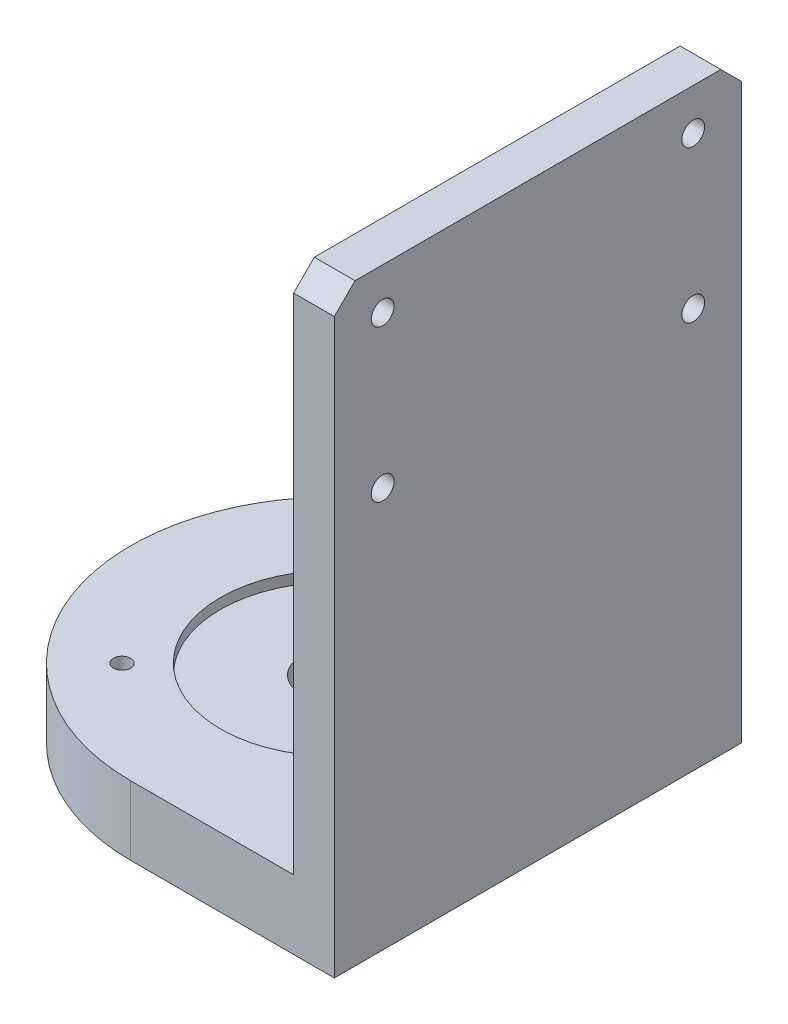
SolidWorks part; units mm, degrees
ref_plane "Front Plane" through (0, 0, 0) normal (0, 0, 1) x (1, 0, 0)
ref_plane "Top Plane" through (0, 0, 0) normal (0, 1, 0) x (1, 0, 0)
ref_plane "Right Plane" through (0, 0, 0) normal (1, 0, 0) x (0, 0, -1)
sketch "Sketch1" plane through (0, 0, 0) normal (0, 0, 1) x (1, 0, 0)
  line L0 (15.9, 0.233) -> (-43.1, 0.233)
  line L1 (0, 86.233) -> (0, 0.233) construction
  line L2 (10, 86.233) -> (10, 10.233)
  line L3 (10, 10.233) -> (-43.1, 10.233)
  line L4 (15.9, 0.233) -> (15.9, 86.233)
  line L5 (15.9, 86.233) -> (10, 86.233)
  line L6 (-43.1, 10.233) -> (-43.1, 0.233)
  line L8 (10, 86.233) -> (10, 0.233) construction
  line L9 (15.9, 10.233) -> (-43.1, 10.233) construction
  dimension "D1" = 59
  dimension "D2" = 86
  dimension "D3" = 15.9
  dimension "D4" = 10
  dimension "D5" = 10
extrude "Boss-Extrude1" add sketch "Sketch1" along normal mid plane 59
sketch "Sketch2" plane through (0, 0.233, 0) normal (0, -1, 0) x (1, 0, 0)
  line L0 (-43.1, 29.5) -> (-43.1, -29.5) construction
  line L1 (-13.6, 29.5) -> (-46.5962, 29.5)
  line L2 (-46.5962, 29.5) -> (-46.5962, -29.5)
  line L3 (-46.5962, -29.5) -> (-13.6, -29.5)
  arc A0 (-13.6, 29.5) -> (-13.6, -29.5) centre (-13.6, 0) ccw
  circle A1 centre (-13.6, 0) radius 4.8
  line M4 (15.9, 29.5) -> (-43.1, 29.5)
  line M5 (-43.1, 29.5) -> (-43.1, -29.5)
  dimension "D1" = 9.6
extrude "Cut-Extrude1" cut sketch "Sketch2" against normal blind 10 contours A0 M4 M5 | A0 L3 M5 | A1
sketch "Sketch4" plane through (0, 10.233, 0) normal (0, 1, 0) x (1, 0, 0)
  circle A0 centre (-13.6, 0) radius 16.5
  dimension "D1" = 33
extrude "Cut-Extrude2" cut sketch "Sketch4" against normal blind 1.5
hole_wizard "M3 Tapped Hole1" positions "Sketch5" profile "Sketch6" tap size "M3" standard "GB" end condition through all
sketch "Sketch5" plane through (0, 10.233, 0) normal (0, 1, 0) x (1, 0, 0)
  point P0 (-28.9796, -15.3796)
  point P4 (-28.9796, 15.3796)
  point P7 (1.7796, 15.3796)
  point P10 (1.7796, -15.3796)
sketch "Sketch6" plane through (-28.9796, 10.233, 15.3796) normal (1, 0, 0) x (0, 0, 1)
  line L0 (0, 0) -> (0, 10)
  line L1 (0, 10) -> (1.25, 10)
  line L2 (1.25, 10) -> (1.25, 0)
  line L5 (1.25, 0) -> (0, 0)
  line L11 (0, -6.35) -> (0, 107.95) construction
  dimension "通孔螺纹孔钻头直径" = 2.5
  dimension "通孔螺纹孔钻头深度" = 10
cosmetic thread "Cosmetic Thread1" parameters "D2"=3
cosmetic thread "Cosmetic Thread2" parameters "D2"=3
cosmetic thread "Cosmetic Thread3" parameters "D2"=3
cosmetic thread "Cosmetic Thread4" parameters "D2"=3
chamfer "Chamfer1" distance 3 angle 45 2 edges at (12.95, 86.233, 29.5) (12.95, 86.233, -29.5)
hole_wizard "M4 Tapped Hole1" positions "Sketch7" profile "Sketch8" tap size "M4" standard "GB" end condition through all
sketch "Sketch7" plane through (10, 0, 0) normal (-1, 0, 0) x (0, 0, 1)
  line L0 (0, 68.2412) -> (0, 94.4251) construction
  line L2 (26.5, 86.233) -> (-26.5, 86.233) construction
  point P0 (-22.5, 80.233)
  point P2 (-22.5, 58.233)
  point P13 (22.5, 58.233)
  point P14 (22.5, 80.233)
  dimension "D1" = 6
  dimension "D2" = 28
  dimension "D3" = 22.5
sketch "Sketch8" plane through (10, 80.233, -22.5) normal (0, 1, 0) x (0, 0, 1)
  line L0 (0, 0) -> (0, 5.9)
  line L1 (0, 5.9) -> (1.65, 5.9)
  line L2 (1.65, 5.9) -> (1.65, 0)
  line L5 (1.65, 0) -> (0, 0)
  line L11 (0, -6.35) -> (0, 107.95) construction
  dimension "通孔螺纹孔钻头直径" = 3.3
  dimension "通孔螺纹孔钻头深度" = 5.9
cosmetic thread "Cosmetic Thread5" parameters "D2"=4
cosmetic thread "Cosmetic Thread6" parameters "D2"=4
cosmetic thread "Cosmetic Thread7" parameters "D2"=4
cosmetic thread "Cosmetic Thread8" parameters "D2"=4
